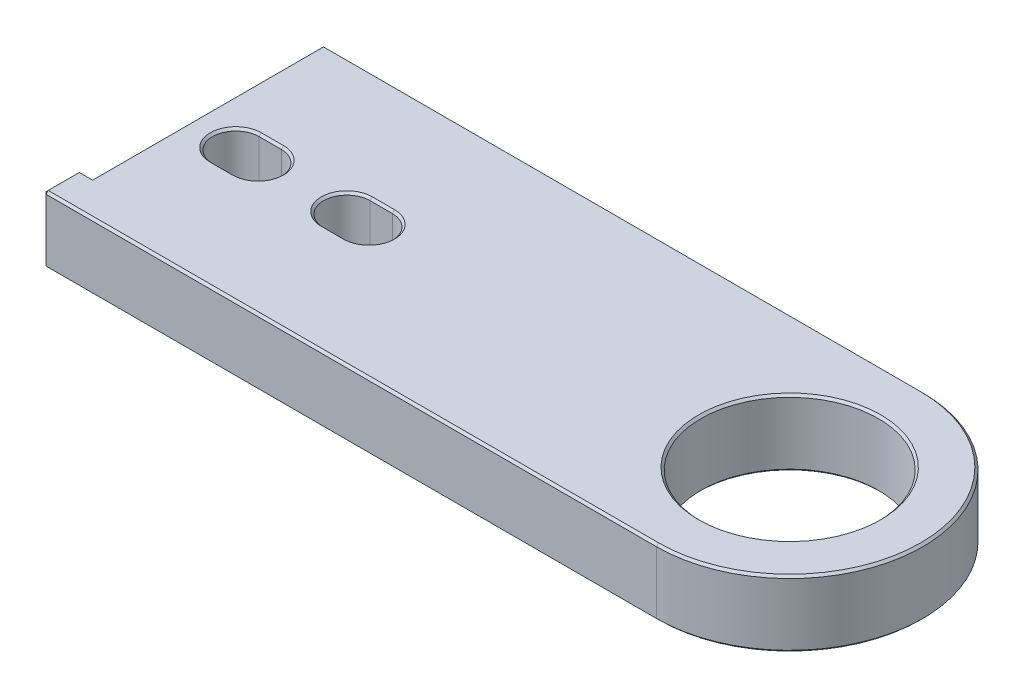
from build123d import *

# Parameters (mm, degrees)
SKETCH_1_R      = 20
EXTRUDE_1_DEPTH = 15
SKETCH_3_W      = 3
SKETCH_3_H      = 8
EXTRUDE_3_DEPTH = 15
CHAMFER_2_SIZE  = 0.5


with BuildPart() as part:
    # 草图1 → 凸台-拉伸1 (new body)
    with BuildSketch(Plane(origin=(0, 0, 0), x_dir=(1, 0, 0), z_dir=(0, 1, 0))):
        with BuildLine():
            Line((-135, 30), (-135, -30))
            Line((-135, -30), (0, -30))
            ThreePointArc((0, -30), (30, 0), (0, 30))
            Line((0, 30), (-135, 30))
        make_face()
        with Locations(Location((0, 0, 0), (0, 0, 270))):
            Circle(SKETCH_1_R, mode=Mode.SUBTRACT)
        with BuildLine():
            Line((-124.75, 5.25), (-119.75, 5.25))
            ThreePointArc((-119.75, 5.25), (-114.5, 0), (-119.75, -5.25))
            Line((-119.75, -5.25), (-124.75, -5.25))
            ThreePointArc((-124.75, -5.25), (-130, 0), (-124.75, 5.25))
        make_face(mode=Mode.SUBTRACT)
        with BuildLine():
            Line((-99.75, 5.25), (-94.75, 5.25))
            ThreePointArc((-94.75, 5.25), (-89.5, 0), (-94.75, -5.25))
            Line((-94.75, -5.25), (-99.75, -5.25))
            ThreePointArc((-99.75, -5.25), (-105, 0), (-99.75, 5.25))
        make_face(mode=Mode.SUBTRACT)
    extrude(amount=EXTRUDE_1_DEPTH)

    # 草图3 → 凸台-拉伸3 (add, through all)
    with BuildSketch(Plane.XZ):
        with Locations((-136.5, 26)):
            Rectangle(SKETCH_3_W, SKETCH_3_H)
    extrude(amount=-EXTRUDE_3_DEPTH)

    # 倒角2
    chamfer_2_edges = [part.edges().sort_by_distance(p)[0] for p in [
        (-67.5, 15, -30),
        (0, 0, -20),
        (0, 15, -20),
        (-135, 15, -4),
        (-130, 0, 0),
        (-122.25, 0, 5.25),
        (-114.5, 0, 0),
        (-122.25, 0, -5.25),
        (-130, 15, 0),
        (-122.25, 15, 5.25),
        (-114.5, 15, 0),
        (-122.25, 15, -5.25),
        (-105, 0, 0),
        (-97.25, 0, 5.25),
        (-89.5, 0, 0),
        (-97.25, 0, -5.25),
        (-105, 15, 0),
        (-97.25, 15, 5.25),
        (-89.5, 15, 0),
        (-97.25, 15, -5.25),
        (-69, 15, 30),
        (-135, 0, -4),
        (-136.5, 15, 22),
        (-138, 15, 26),
        (-138, 7.5, 22),
        (-138, 7.5, 30),
        (-67.5, 0, -30),
        (-138, 0, 26),
        (-136.5, 0, 22),
        (30, 0, 0),
        (-69, 0, 30),
        (30, 15, 0),
        (-135, 7.5, -30),
    ]]
    chamfer(chamfer_2_edges, length=CHAMFER_2_SIZE)


solid = part.part
